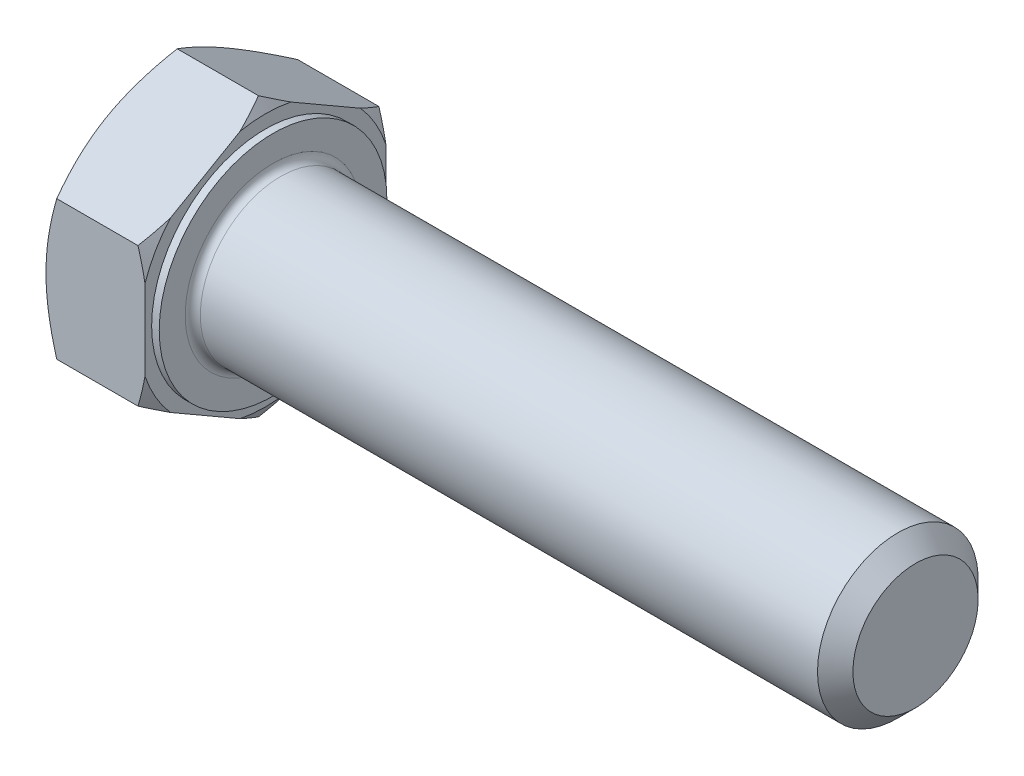
SolidWorks part; units mm, degrees
material "SAE5"
ref_plane "Front Plane" through (0, 0, 0) normal (0, 0, 1) x (1, 0, 0)
ref_plane "Top Plane" through (0, 0, 0) normal (0, 1, 0) x (1, 0, 0)
ref_plane "Right Plane" through (0, 0, 0) normal (1, 0, 0) x (0, 0, -1)
sketch "Sketch1" plane through (0, 0, 0) normal (1, 0, 0) x (0, 0, -1)
  line L0 (9.525, 5.4993) -> (9.525, -5.4993)
  line L1 (-9.525, 5.4993) -> (-9.525, -5.4993)
  line L2 (9.525, -5.4993) -> (0, -10.9985)
  line L3 (0, -10.9985) -> (-9.525, -5.4993)
  line L4 (9.525, 5.4993) -> (0, 10.9985)
  line L5 (0, 10.9985) -> (-9.525, 5.4993)
  dimension "s" = 19.05
  dimension "D2" = 120
  dimension "D3" = 9.525
  dimension "D4" = 9.525
  dimension "D5" = 9.525
extrude "Base-Extrude" add sketch "Sketch1" along normal blind 8.7312
sketch "Sketch2" plane through (0, 0, 0) normal (0, 0, 1) x (1, 0, 0)
  line L0 (0, 5.4993) -> (0, -5.4993) construction
  line L1 (0, 0) -> (59.5312, 0)
  line L2 (0, 0) -> (0, 6.35)
  line L3 (0, 6.35) -> (27.8072, 6.35)
  line L4 (59.5312, 0) -> (59.5312, 5.5562)
  line L5 (8.7312, 10.9985) -> (8.7312, 5.4993) construction
  line L7 (0, 0) -> (96.52, 0) construction
  line L8 (59.5312, -5.5562) -> (27.8072, -6.35) construction
  line L9 (0, -6.35) -> (27.8072, -6.35) construction
  line L10 (10.4812, 15.24) -> (10.4813, -1.27) construction
  line L11 (27.7812, 15.24) -> (27.7812, -1.27) construction
  line L12 (8.7312, 5.4993) -> (8.7312, -5.4993) construction
  line L13 (27.8072, 6.35) -> (59.5312, 6.35)
  line L14 (59.5312, 6.35) -> (59.5312, 5.5562)
  dimension "l" = 50.8
  dimension "m" = 12.7
  dimension "Minor_dia" = 11.1125
  dimension "p" = 1.75
  dimension "h" = 31.75
revolve "Boss-Revolve1" add sketch "Sketch2" angle 360 about L7
cosmetic thread "Helix1" parameters "Thread_length"=30, "Thread_minor"=8.969
sketch "Sketch3" plane through (0, 0, 0) normal (0, 0, 1) x (1, 0, 0)
  line L0 (0, 9) -> (4.0406, 15.9985)
  line L1 (0, 10.9985) -> (0, 5.4993) construction
  line L2 (4.0406, 15.9985) -> (4.0406, 20.9985)
  line L3 (4.0406, 20.9985) -> (-10, 20.9985)
  line L4 (-10, 20.9985) -> (-10, 9)
  line L5 (-10, 9) -> (0, 9)
  line L6 (0, 0) -> (99.06, 0) construction
  line L7 (8.7312, 10.9985) -> (0, 10.9985) construction
  dimension "D1" = 9
  dimension "D2" = 5
  dimension "D3" = 10
  dimension "D4" = 5
  dimension "Head_ch_ang" = 30
revolve "Cut-Revolve1" cut sketch "Sketch3" angle 360 about L6
sketch "Sketch5" plane through (0, 0, 0) normal (0, 0, 1) x (1, 0, 0)
  line L0 (8.7312, 9) -> (4.6907, 15.9985)
  line L1 (8.7312, 10.9985) -> (8.7312, 5.4993) construction
  line L2 (4.6907, 15.9985) -> (4.6907, 20.9985)
  line L3 (4.6907, 20.9985) -> (14.6907, 20.9985)
  line L4 (14.6907, 20.9985) -> (14.6907, 9)
  line L5 (14.6907, 9) -> (8.7312, 9)
  line L7 (8.7312, 10.9985) -> (1.1538, 10.9985) construction
  line L8 (0, 0) -> (99.06, 0) construction
  line L9 (0, 0) -> (99.06, 0) construction
  dimension "D1" = 9
  dimension "D2" = 5
  dimension "D3" = 10
  dimension "Head_ch_ang" = 30
  dimension "D4" = 5
revolve "Cut-Revolve2" cut sketch "Sketch5" angle 360 about L8
sketch "Sketch4" plane through (0, 0, 0) normal (0, 0, 1) x (1, 0, 0)
  line L1 (8.7312, 10.9985) -> (8.7312, 5.4993) construction
  line L2 (8.7312, 9) -> (8.1312, 9)
  line L3 (8.7312, 9) -> (8.7312, 20.9985)
  line L4 (8.7312, 20.9985) -> (8.1312, 20.9985)
  line L5 (0, 0) -> (95.25, 0) construction
  line L6 (0, 0) -> (96.52, 0) construction
  line L7 (8.1312, 9) -> (8.1312, 20.9985)
  line L8 (7.5774, 10.9985) -> (1.1538, 10.9985) construction
  dimension "D1" = 18
  dimension "D2" = 10
  dimension "c" = 0.6
revolve "Cut-Revolve3" cut sketch "Sketch4" angle 360 about L5
chamfer "Chamfer" distance 1.4 angle 45 1 edges at (59.5312, 0, 6.35)
fillet "Fillet" radius 0.6 1 edges at (8.7312, 0, -6.35)
sketch "Sketch6" plane through (0, 0, 0) normal (0, 0, 1) x (1, 0, 0)
  line L0 (77.5, -4.4845) -> (76.625, -6)
  line L1 (77.5, -4.4845) -> (78.375, -6)
  line L2 (78.375, -6) -> (78.375, -7.5)
  line L3 (-3.175, 0) -> (5.1513, 0) construction
  line L5 (78.375, -7.5) -> (76.625, -7.5)
  line L6 (76.625, -7.5) -> (76.625, -6)
  dimension "Thread_minor" = 8.969
  dimension "Diameter" = 12
  dimension "Start" = 77.5
  dimension "SideAngle" = 60
  dimension "VeeAngle" = 60
  dimension "Overcut" = 15
revolve "Cut-Revolve4" [suppressed] cut sketch "Sketch6" angle 360 about L3
pattern_linear "LPattern1" [suppressed]
